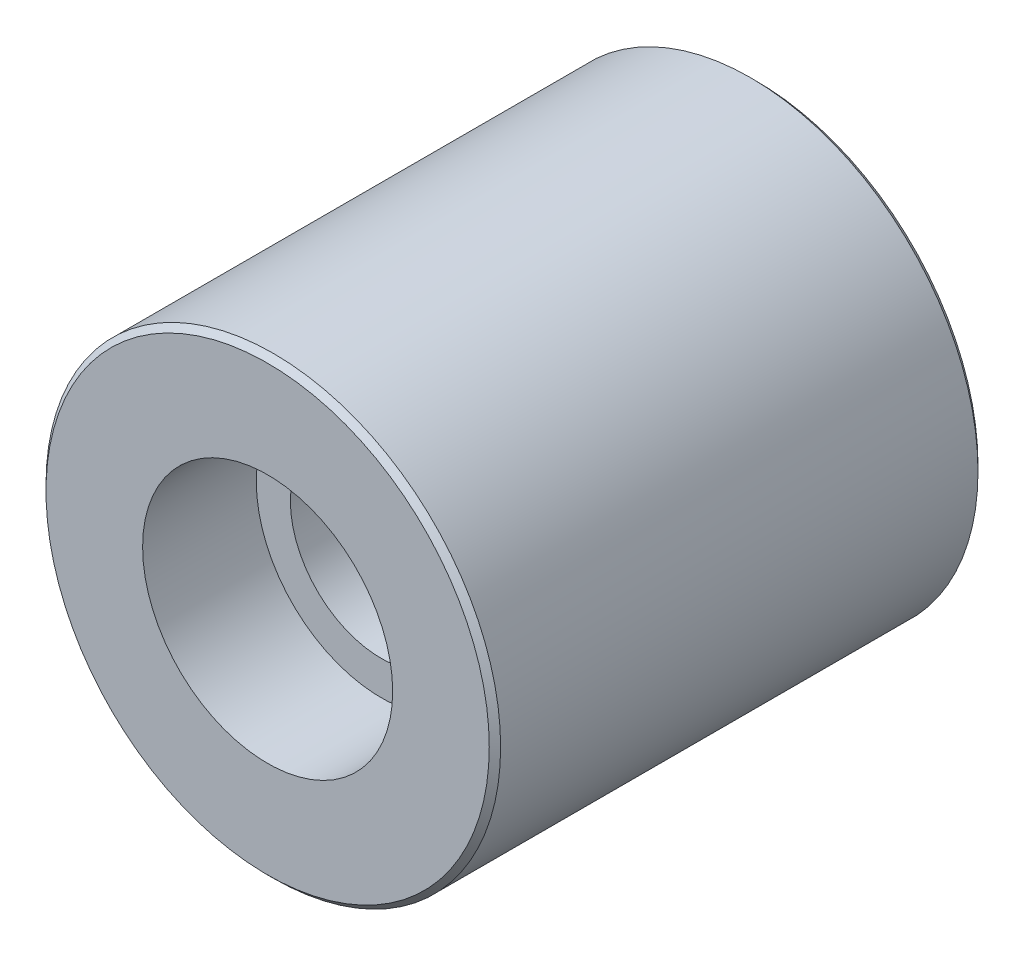
SolidWorks part; units mm, degrees
ref_plane "前视基准面" through (0, 0, 0) normal (0, 0, 1) x (1, 0, 0)
ref_plane "上视基准面" through (0, 0, 0) normal (0, 1, 0) x (1, 0, 0)
ref_plane "右视基准面" through (0, 0, 0) normal (1, 0, 0) x (0, 0, -1)
sketch "草图1" plane through (0, 0, 0) normal (0, 0, 1) x (1, 0, 0)
  circle A0 centre (0, 0) radius 20
  dimension "D1" = 40
extrude "凸台-拉伸1" add sketch "草图1" along normal blind 43
sketch "草图2" plane through (0, 0, 43) normal (0, 0, 1) x (1, 0, 0)
  circle A0 centre (0, 0) radius 11
  dimension "D1" = 22
extrude "切除-拉伸1" cut sketch "草图2" against normal blind 10
sketch "草图3" plane through (0, 0, 0) normal (0, 0, -1) x (-1, 0, 0)
  circle A0 centre (0, 0) radius 11
  dimension "D1" = 22
extrude "切除-拉伸2" cut sketch "草图3" against normal blind 7
sketch "草图4" plane through (0, 0, 7) normal (0, 0, -1) x (-1, 0, 0)
  circle A0 centre (0, 0) radius 8
  dimension "D1" = 16
extrude "切除-拉伸3" cut sketch "草图4" against normal through all
chamfer "倒角1" distance 0.5 angle 45 2 edges at (20, 0, 0) (20, 0, 43)
